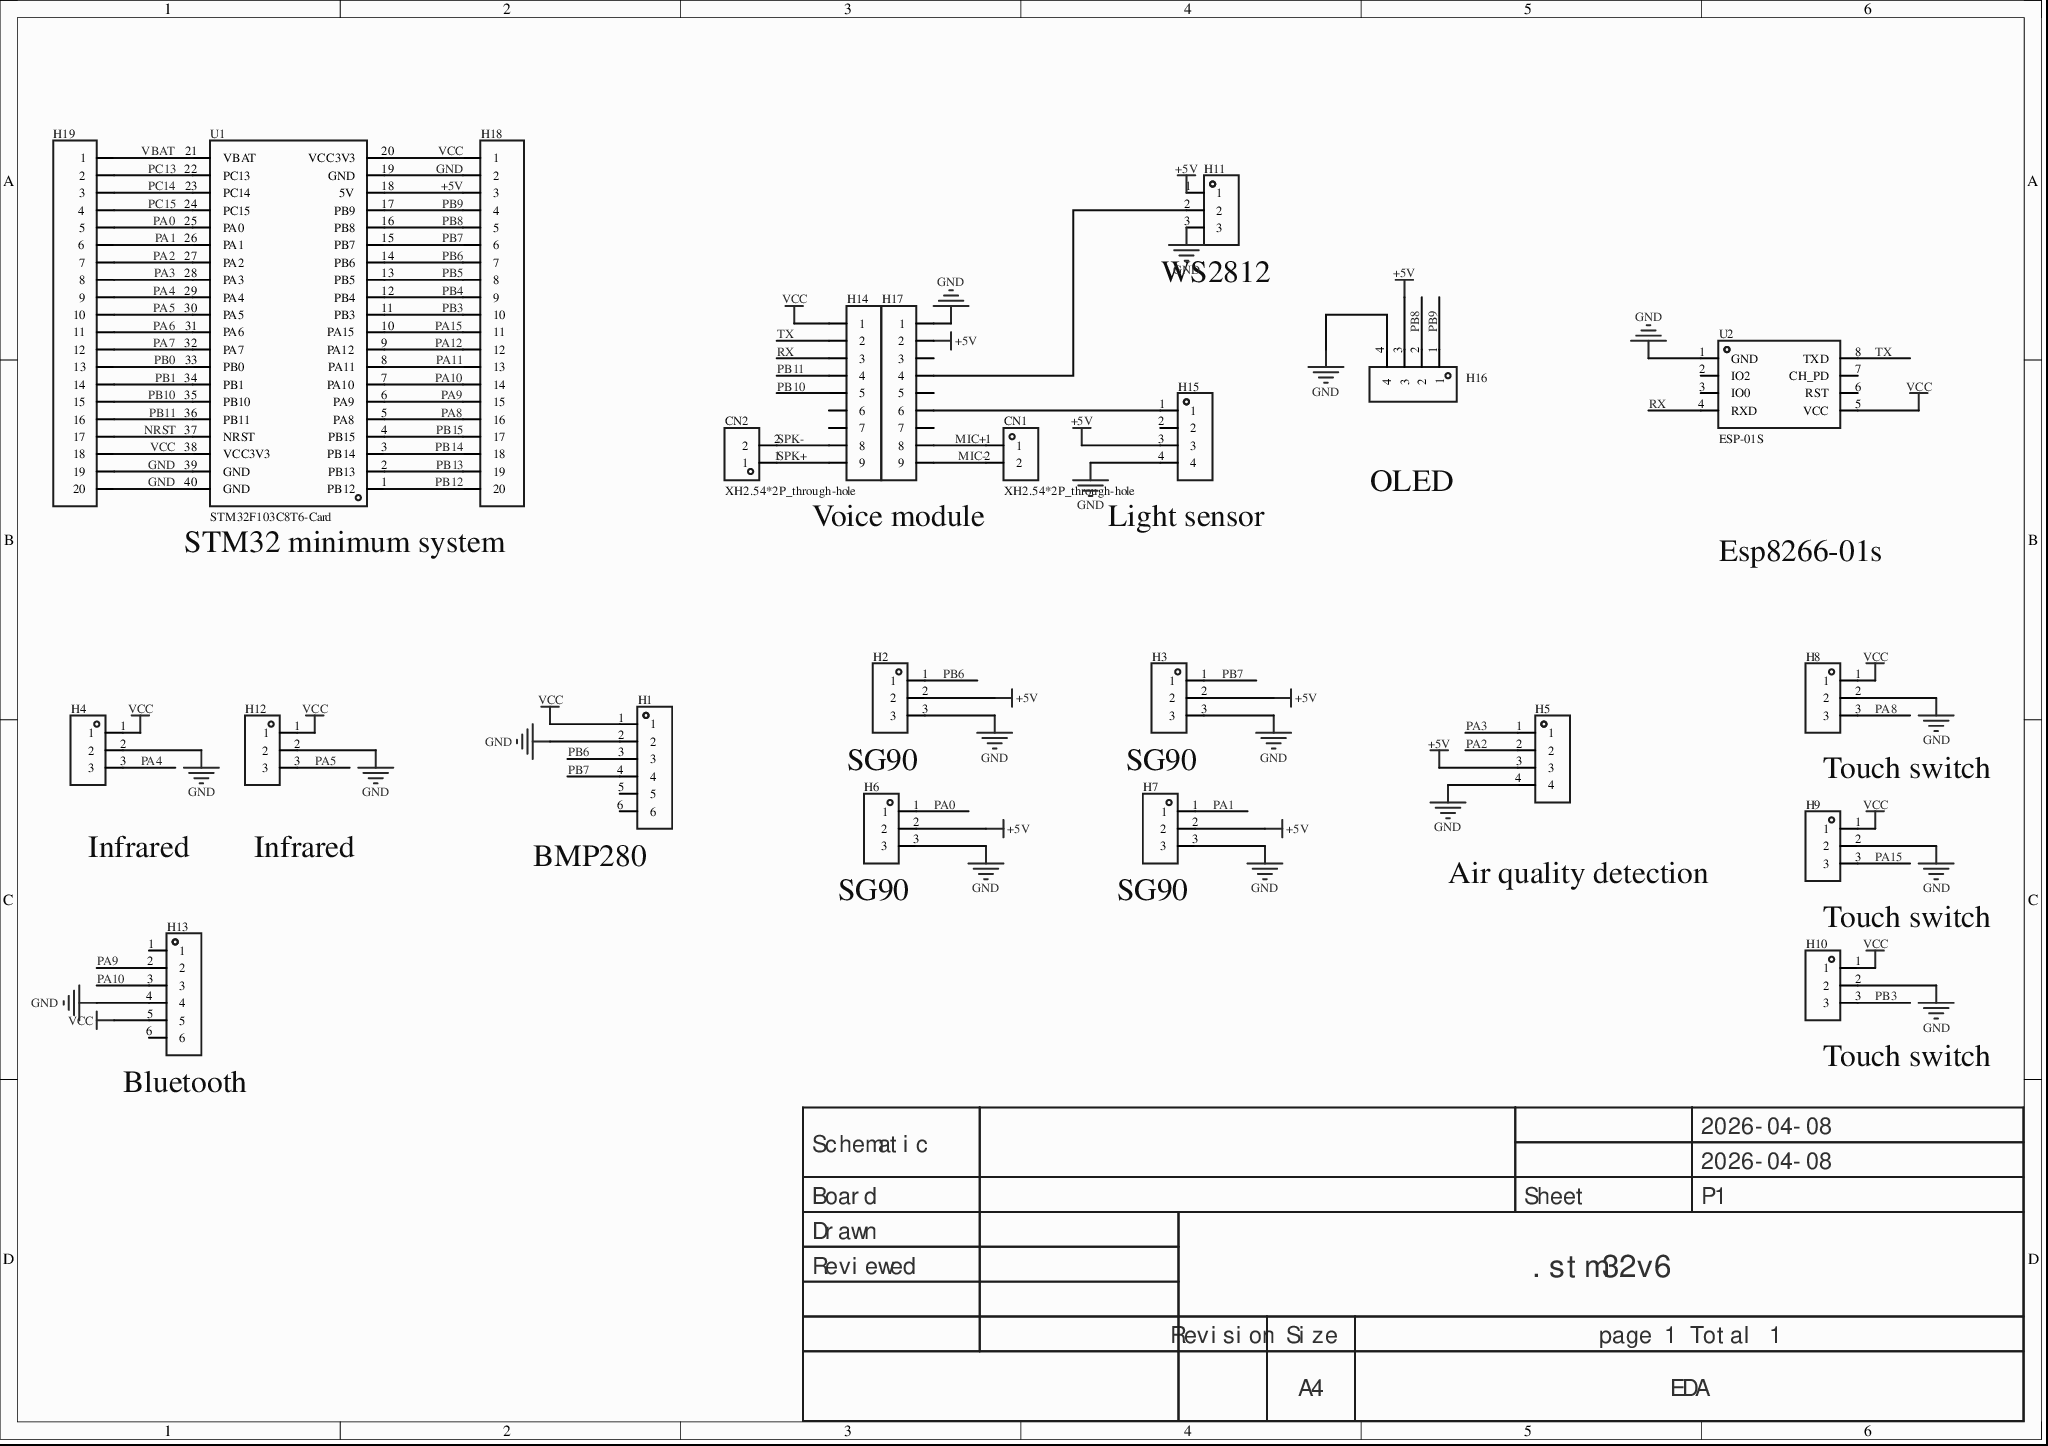
[diagram p0: MISC51613-3.schdoc]
# Altium project MISC51613-2.PrjPcb
1 sheet, 23 parts. Net scope: global (net labels, ports and power ports of the same name join across sheets).
Board file: MISC51613.pcbdoc

## Sheet MISC51613-3.schdoc
size 297 x 209 mm; Version: V1.0; @Project Name: MISC51613; @Page Count: 1; @Update Date: 2026-04-08; @Create Date: 2026-04-08; @Schematic Name: MISC51613; @Page No: 1; @Create Time: 23:22:16; @Update Time: 17:32:40; @Board Name: MISC51613

### Parts
CN1  XH2.54*2P_through-hole  [CONN-TH_2P-P2.50-XH2.54-2P]
CN2  XH2.54*2P_through-hole  [CONN-TH_2P-P2.50-XH2.54-2P]
H1  (no value)  [HDR-TH_6P-P2.54-V-F]
H2  (no value)  [HDR-TH_3P-P2.54-V-F]
H3  (no value)  [HDR-TH_3P-P2.54-V-F]
H4  (no value)  [HDR-TH_3P-P2.54-V-F]
H5  (no value)  [HDR-TH_4P-P2.54-V-F]
H6  (no value)  [HDR-TH_3P-P2.54-V-F]
H7  (no value)  [HDR-TH_3P-P2.54-V-F]
H8  (no value)  [HDR-TH_3P-P2.54-V-F]
H9  (no value)  [HDR-TH_3P-P2.54-V-F]
H10  (no value)  [HDR-TH_3P-P2.54-V-F]
H11  (no value)  [HDR-TH_3P-P2.54-V-F]
H12  (no value)  [HDR-TH_3P-P2.54-V-F]
H13  (no value)  [HDR-TH_6P-P2.54-V-F]
H14  (no value)  [HDR-TH_9P-P2.54-V-F-1]
H15  (no value)  [HDR-TH_4P-P2.54-V-F]
H16  (no value)  [HDR-TH_4P-P2.54-V-F]
H17  (no value)  [HDR-TH_9P-P2.54-V-F-1]
H18  (no value)  [HDR-TH_20P-P2.54-V-F]
H19  (no value)  [HDR-TH_20P-P2.54-V-F]
U1  STM32F103C8T6-Card  [CONN-TH_L53.3-W22.9_STM32F103C8T6-CARD]
U2  ESP-01S  [WIFIM-TH_ESP-01S]

### Nets
+5V: H2.2 H3.2 H5.3 H6.2 H7.2 H11.1 H15.3 H16.3 H17.2 H18.3 U1.18(5V)
GND: H1.2 H2.3 H3.3 H4.2 H5.4 H6.3 H7.3 H8.2 H9.2 H10.2 H11.3 H12.2 H13.4 H15.4 H16.4 H17.1 H18.2 H19.19 H19.20 U1.19(GND) U1.39(GND) U1.40(GND) U2.1(GND)
VCC: H1.1 H4.1 H8.1 H9.1 H10.1 H12.1 H13.5 H14.1 H18.1 H19.18 U1.20(VCC3V3) U1.38(VCC3V3) U2.5(VCC)
MIC+: CN1.1 H17.8
MIC-: CN1.2 H17.9
NRST: H19.17 U1.37(NRST)
PA0: H6.1 H19.5 U1.25(PA0)
PA1: H7.1 H19.6 U1.26(PA1)
PA2: H5.2 H19.7 U1.27(PA2)
PA3: H5.1 H19.8 U1.28(PA3)
PA4: H4.3 H19.9 U1.29(PA4)
PA5: H12.3 H19.10 U1.30(PA5)
PA6: H19.11 U1.31(PA6)
PA7: H19.12 U1.32(PA7)
PA8: H8.3 H18.16 U1.5(PA8)
PA9: H13.2 H18.15 U1.6(PA9)
PA10: H13.3 H18.14 U1.7(PA10)
PA11: H18.13 U1.8(PA11)
PA12: H18.12 U1.9(PA12)
PA15: H9.3 H18.11 U1.10(PA15)
PB0: H19.13 U1.33(PB0)
PB1: H19.14 U1.34(PB1)
PB3: H10.3 H18.10 U1.11(PB3)
PB4: H18.9 U1.12(PB4)
PB5: H18.8 U1.13(PB5)
PB6: H1.3 H2.1 H18.7 U1.14(PB6)
PB7: H1.4 H3.1 H18.6 U1.15(PB7)
PB8: H16.2 H18.5 U1.16(PB8)
PB9: H16.1 H18.4 U1.17(PB9)
PB10: H14.5 H19.15 U1.35(PB10)
PB11: H14.4 H19.16 U1.36(PB11)
PB12: H18.20 U1.1(PB12)
PB13: H18.19 U1.2(PB13)
PB14: H18.18 U1.3(PB14)
PB15: H18.17 U1.4(PB15)
PC13: H19.2 U1.22(PC13)
PC14: H19.3 U1.23(PC14)
PC15: H19.4 U1.24(PC15)
RX: H14.3 U2.4(RXD)
SPK+: CN2.1 H14.9
SPK-: CN2.2 H14.8
TX: H14.2 U2.8(TXD)
VBAT: H19.1 U1.21(VBAT)
NetH11_2: H11.2 H17.4
NetH15_1: H15.1 H17.6

Not connected (* = marked no-connect by the designer): H1 5 6; H13 1 6; H14 6 7; H15 2; H17 3 5 7; U2 2(IO2)* 3(IO0)* 6(RST)* 7(CH_PD)*

### Notes on the sheet
- (near H11) WS2812
- OLED
- STM32 minimum system
- Voice module
- (near H15) Light sensor
- Esp8266-01s
- SG90
- Touch switch
- Infrared
- (near H12) Infrared
- (near H1) BMP280
- (near H6) SG90
- (near H7) SG90
- Air quality detection
- (near H13) Bluetooth
- (near H10) Touch switch
- 2026-04-08
- Schematic
- Board
- Sheet
- P1
- Drawn
- Reviewed
- .stm32v6
- Revision
- Size
- A4
- page 1 Total 1
- EDA

### Library data of the parts
CN1 CN2 = XH2.54*2P_直插: AddInBom: yes; ModelId: 325c595e30db4df8abe76612dd40b0fa0819f05c4eef4c71ace90d822a990e87; ModelTransform: 295.275,228.346,0,180,0,0,-0.002,-20.079,-137.795; Symbol: XH2.54*2P_through-hole; Device: XH2.54*2P_through-hole; LCSC Part Name: XH2.54*2P_直插; SupplierPart: C9900008615; ManufacturerPart: XH2.54*2P_直插; Supplier Footprint: XH2.54_2P; JLCPCB Part Class: Extended Part; Supplier: LCSC; ConvertToPcb: yes; FootprintName: CONN-TH_2P-P2.50-XH2.54-2P; ModelName: CONN-TH_2P-P2.50-XH2.54-2P
H1 H13 = HDR-F_2.54_1x6P: Symbol: Header-Female-2.54_1x6; ConvertToPcb: yes; ModelId: 0f5bcf94dcda47d085f24cdca1696fe9; ModelTransform: 619.684,94.488,0,0,0,0,0,0,-125.984; Device: HDR-F_2.54_1x6P; AddInBom: yes; SupplierPart: C40877; Supplier Footprint: 插件; FootprintName: HDR-TH_6P-P2.54-V-F; ModelName: HDR-TH_6P-P2.54-V-F
H2-H4 H6-H12 = HDR-F_2.54_1x3P: Symbol: PM254V-11-03-H85; 3D Model: f3b3cc5aae9641bf9e56fc160cef875b; 3D Model Transform: 299.9994,100,0,0,0,0,0,0,-118.11; ConvertToPcb: yes; ModelName: HDR2.54-F-LI-1X3P; Device: HDR-F_2.54_1x3P; Supplier Part: C541850; Supplier Footprint: 插件; AddInBom: yes; FootprintName: HDR-TH_3P-P2.54-V-F
H5 H15 H16 = HDR-F_2.54_1x4P: Symbol: 2.54-1*4P female; ConvertToPcb: yes; ModelId: d187812051054f85879fcaa51a310d8e0819f05c4eef4c71ace90d822a990e87; ModelTransform: 419.6842,98.464,0,0,0,0,0,0,-118.11; Device: HDR-F_2.54_1x4P; AddInBom: yes; SupplierPart: C2718488; Supplier Footprint: 插件; FootprintName: HDR-TH_4P-P2.54-V-F; ModelName: HDR-TH_4P-P2.54-V-F
H14 H17 = HDR-F_2.54_1x9P: Symbol: Header-Female-2.54_1x9; AddInBom: yes; ModelId: 3a7016416d904017ac5ead6cc0f14e9c0819f05c4eef4c71ace90d822a990e87; ModelName: HDR-TH_9P-P2.54-F-LI-1X9P; ModelTransform: 915.746,94.488,0,0,0,0,0,0,-125.984; Device: HDR-F_2.54_1x9P; ConvertToPcb: yes; FootprintName: HDR-TH_9P-P2.54-V-F-1; SupplierPart: C39576; Supplier Footprint: 插件
H18 H19 = HDR-F_2.54_1x20P: ConvertToPcb: yes; ModelId: db7015f7ad9d48b8a3b1188db02e3429; ModelName: HDR-F-2.54_1x20; ModelTransform: 1999.996,100,0,0,0,0,0,0,-118.11; Symbol: HDR-F_2.54_1x20P; Device: HDR-F_2.54_1x20P; AddInBom: yes; SupplierPart: C50984; Supplier Footprint: 插件; FootprintName: HDR-TH_20P-P2.54-V-F
U1 = STM32F103C8T6-Card: AddInBom: yes; Symbol: STM32F103C8T6-CARD; Device: STM32F103C8T6-Card; LCSC Part Name: STM32F103C8T6-Card; SupplierPart: C9900077949; ManufacturerPart: STM32F103C8T6-Card; Supplier Footprint: 插件; Supplier: LCSC; ConvertToPcb: yes; FootprintName: CONN-TH_L53.3-W22.9_STM32F103C8T6-CARD
U2 = ESP-01S_C111009: AddInBom: yes; ModelId: eb7175da78ae48b3b1568cfe3027405f0819f05c4eef4c71ace90d822a990e87; ModelTransform: 582.676,976.37608,0,0,0,0,0,388.346,-118.11; Symbol: ESP-01S; Device: ESP-01S_C111009; LCSC Part Name: ESP-01S; SupplierPart: C111009; ManufacturerPart: ESP-01S; Supplier Footprint: -; JLCPCB Part Class: Extended Part; Supplier: LCSC; ConvertToPcb: yes; FootprintName: WIFIM-TH_ESP-01S; ModelName: WIFIM-TH_ESP-01S